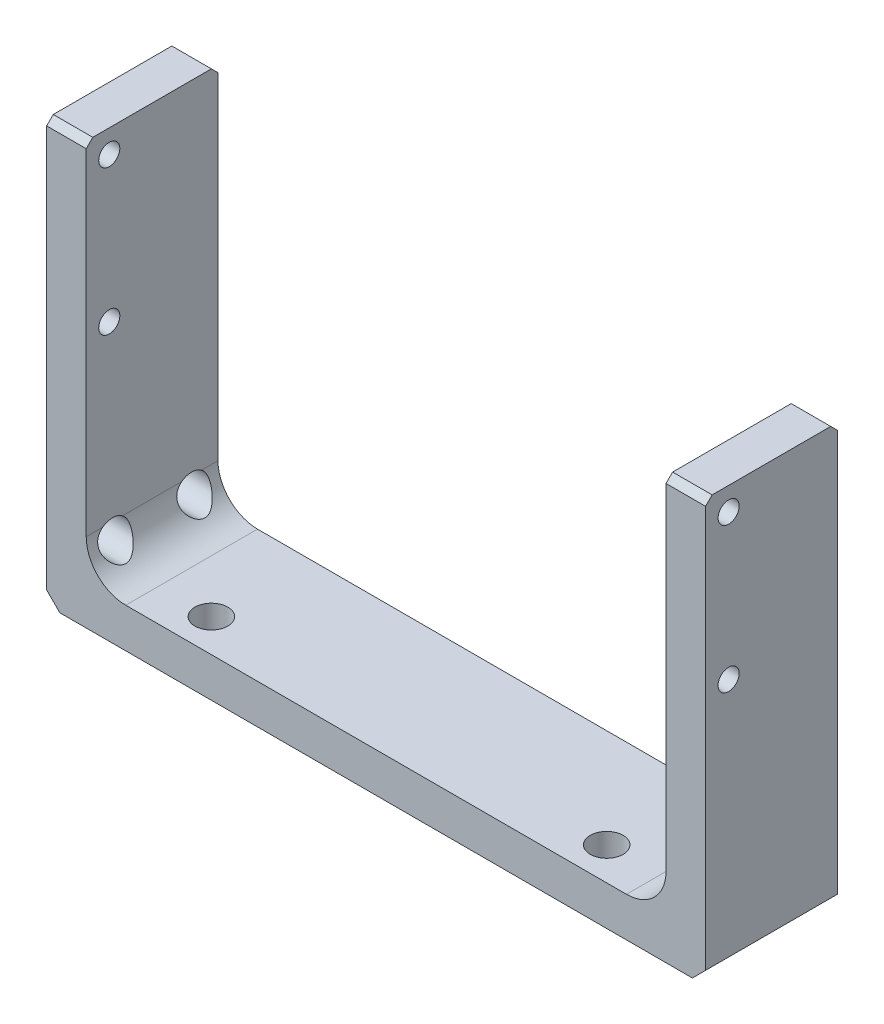
from build123d import *

# Parameters (mm, degrees)
SKETCH26_W                 = 50
SKETCH26_H                 = 32
BOSS_EXTRUDE2_DEPTH        = 5
SKETCH27_W                 = 44
SKETCH27_H                 = 29
CUT_EXTRUDE5_DEPTH         = 32.320919527
FILLET1_R                  = 3
CHAMFER1_SIZE              = 0.5
CHAMFER2_SIZE              = 1
M2_TAPPED_HOLE1_D          = 1.6
F_2_5_2_5_DIAMETER_HOLE1_D = 2.5
M3_TAPPED_HOLE2_REACH      = 54.735
M3_TAPPED_HOLE2_BORE_R     = 1.25


with BuildPart() as part:
    # Sketch26 → Boss-Extrude2 (new, symmetric)
    with BuildSketch(Plane.XY):
        Rectangle(SKETCH26_W, SKETCH26_H)
    extrude(amount=BOSS_EXTRUDE2_DEPTH, both=True)

    # Sketch27 → Cut-Extrude5 (cut, through all)
    with BuildSketch(Plane.XY.offset(5)):
        with Locations((0, 1.5)):
            Rectangle(SKETCH27_W, SKETCH27_H)
    extrude(amount=-CUT_EXTRUDE5_DEPTH, mode=Mode.SUBTRACT)

    # Fillet1
    fillet1_edges = [part.edges().sort_by_distance(p)[0] for p in [
        (22, -13, 0),
        (-22, -13, 0),
    ]]
    fillet(fillet1_edges, radius=FILLET1_R)

    # Chamfer1
    chamfer1_edges = [part.edges().sort_by_distance(p)[0] for p in [
        (-23.5, 16, -5),
        (-23.5, 16, 5),
        (23.5, 16, -5),
        (23.5, 16, 5),
    ]]
    chamfer(chamfer1_edges, length=CHAMFER1_SIZE)

    # Chamfer2
    chamfer2_edges = [part.edges().sort_by_distance(p)[0] for p in [
        (25, -16, 0),
        (-25, -16, 0),
    ]]
    chamfer(chamfer2_edges, length=CHAMFER2_SIZE)

    # M2 Tapped Hole1 (through all)
    with Locations(Plane(origin=(25, 0, 0), x_dir=(0, 0, -1), z_dir=(1, 0, 0))):
        with Locations((-3.25, 14.25), (-3.25, 3.25)):
            Hole(M2_TAPPED_HOLE1_D / 2)

    # Ø2.5 (2.5) Diameter Hole1 (through all)
    with Locations(Plane(origin=(0, -16, 0), x_dir=(-1, 0, 0), z_dir=(0, -1, 0))):
        with Locations((15, -2.5), (-15, -2.5)):
            Hole(F_2_5_2_5_DIAMETER_HOLE1_D / 2)

    # M3 Tapped Hole2 bore → M3 Tapped Hole2 (cut, up to next)
    with BuildSketch(Plane.ZY.offset(25), mode=Mode.PRIVATE) as m3_tapped_hole2_sk1:
        with Locations((-3, -11)):
            Circle(M3_TAPPED_HOLE2_BORE_R)
    m3_tapped_hole2_tool1 = extrude(m3_tapped_hole2_sk1.sketch, amount=-M3_TAPPED_HOLE2_REACH, mode=Mode.PRIVATE) & part.part
    # M3 Tapped Hole2 bore → M3 Tapped Hole2 (cut, up to next)
    with BuildSketch(Plane.ZY.offset(25), mode=Mode.PRIVATE) as m3_tapped_hole2_sk2:
        with Locations((3, -11)):
            Circle(M3_TAPPED_HOLE2_BORE_R)
    m3_tapped_hole2_tool2 = extrude(m3_tapped_hole2_sk2.sketch, amount=-M3_TAPPED_HOLE2_REACH, mode=Mode.PRIVATE) & part.part
    add(m3_tapped_hole2_tool1.solids().sort_by_distance((-25, -11, -3))[0], mode=Mode.SUBTRACT)
    add(m3_tapped_hole2_tool2.solids().sort_by_distance((-25, -11, 3))[0], mode=Mode.SUBTRACT)


solid = part.part
